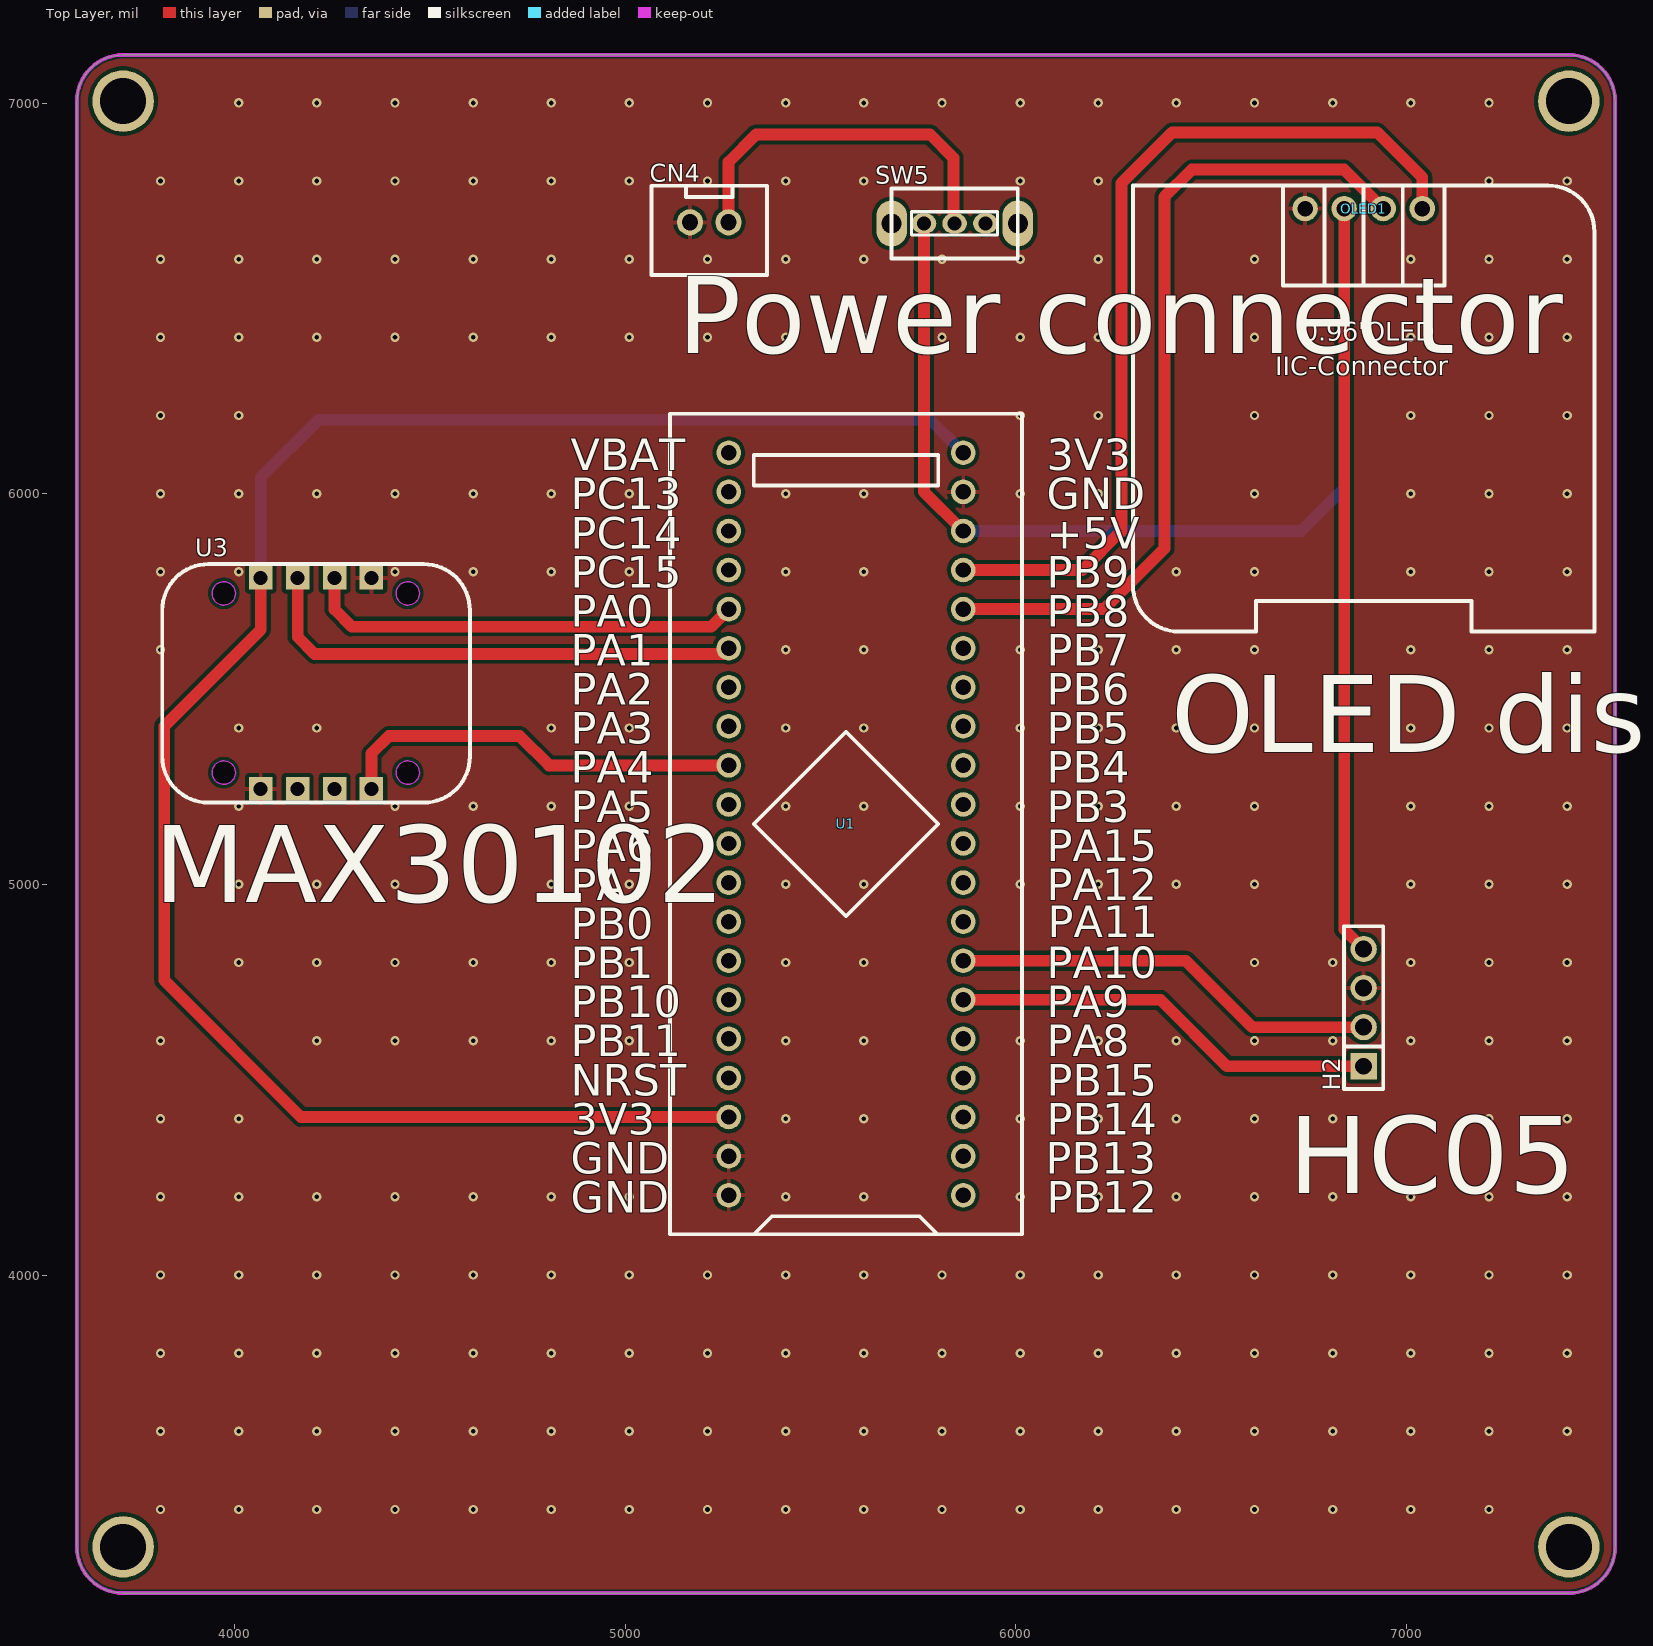
[diagram p0: Top Layer view]
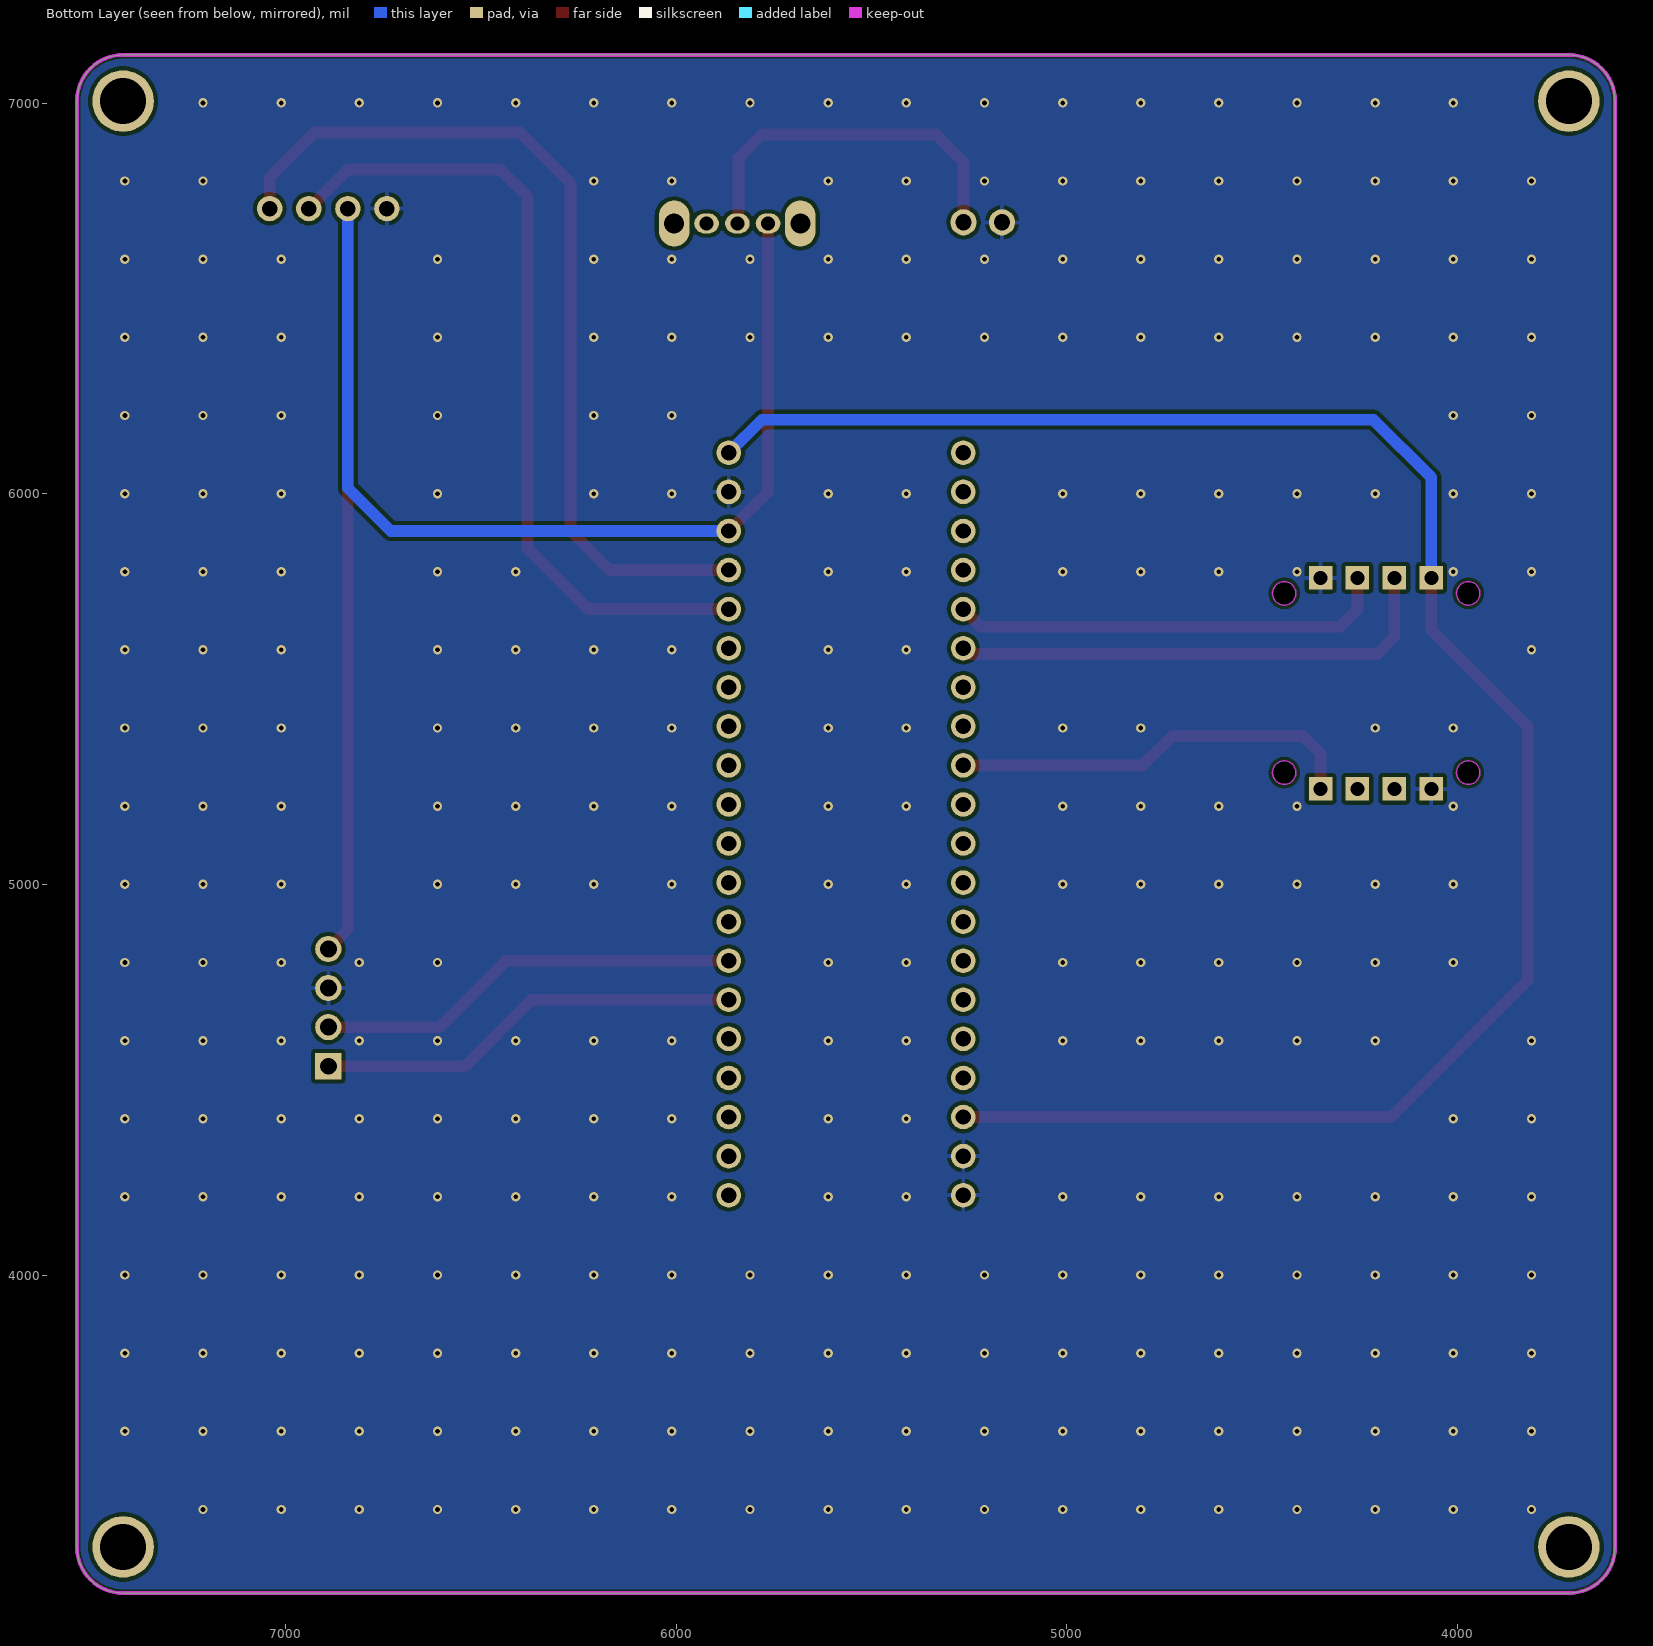
[diagram p1: Bottom Layer view, seen from below]
# Altium PCB MISC50728.pcbdoc
Units mil, origin at the board's own origin, x right, y up, seen from the top; angles counter-clockwise.
Board outline 3937.01 x 3937.01 mil, 2 copper layers (Top Layer, Bottom Layer), stack 62.206 mil thick; 6 components, 38 nets, 67 pads, 286 vias.

## Layer stack, top to bottom
Top Solder Mask Layer: solder mask 0.394, Dk 3.3
Top Layer: signal copper 1.379
Dielectric1: surface 59.449, FR4, Dk 4.5
Bottom Layer: signal copper 1.378
Bottom Solder Mask Layer: solder mask 0.394, Dk 3.3

## Board outline
3714.61,7123.5 ccw(c3714.61,7005.39) 3596.5,7005.39 3596.5,3304.61 ccw(c3714.61,3304.61) 3714.61,3186.5 7415.39,3186.5 ccw(c7415.39,3304.61) 7533.5,3304.61 7533.5,7005.39 ccw(c7415.39,7005.39) 7415.39,7123.5 3714.61,7123.5

## Design rules (kind name [scope] priority, off if disabled: settings)
BoardOutlineClearance copperThickness2oz_1 [All] p2 off: genericclearance=7.99 ignorepadtopadclearanceinfootprint=FALSE except(0: Arc-SplitContinuation Track-SplitContinuation SMDPad-SplitContinuation THPad-SplitContinuation Via-SplitContinuation Fill-SplitContinuation Region-SplitContinuation Poly-SplitContinuation Text-SplitContinuation Hole-SplitContinuation; 5.98: Arc-CutoutEdge Track-CutoutEdge SMDPad-CutoutEdge THPad-CutoutEdge Via-CutoutEdge Text-CutoutEdge; 6.9: Hole-OutlineEdge Hole-CutoutEdge; 10: Poly-OutlineEdge Poly-CutoutEdge; 11.81: Arc-OutlineEdge Track-OutlineEdge SMDPad-OutlineEdge THPad-OutlineEdge Via-OutlineEdge Fill-OutlineEdge Region-OutlineEdge Text-OutlineEdge Fill-CutoutEdge Region-CutoutEdge)
BoardOutlineClearance Plane_innerPlane_1 [All] p4 off: genericclearance=4.02 ignorepadtopadclearanceinfootprint=FALSE except(0: Arc-SplitContinuation Track-SplitContinuation SMDPad-SplitContinuation THPad-SplitContinuation Via-SplitContinuation Fill-SplitContinuation Region-SplitContinuation Poly-SplitContinuation Text-SplitContinuation Hole-SplitContinuation; 5.98: Arc-CutoutEdge Track-CutoutEdge SMDPad-CutoutEdge THPad-CutoutEdge Via-CutoutEdge Text-CutoutEdge; 6.9: Hole-OutlineEdge Hole-CutoutEdge; 10: Poly-OutlineEdge Poly-CutoutEdge; 11.81: Arc-OutlineEdge Track-OutlineEdge SMDPad-OutlineEdge THPad-OutlineEdge Via-OutlineEdge Fill-OutlineEdge Region-OutlineEdge Text-OutlineEdge Fill-CutoutEdge Region-CutoutEdge)
BoardOutlineClearance Copper_copperRegion_1 [All] p6 off: genericclearance=4.02 ignorepadtopadclearanceinfootprint=FALSE except(0: Arc-SplitContinuation Track-SplitContinuation SMDPad-SplitContinuation THPad-SplitContinuation Via-SplitContinuation Fill-SplitContinuation Region-SplitContinuation Poly-SplitContinuation Text-SplitContinuation Hole-SplitContinuation; 5.98: Arc-CutoutEdge Track-CutoutEdge SMDPad-CutoutEdge THPad-CutoutEdge Via-CutoutEdge Text-CutoutEdge; 6.9: Hole-OutlineEdge Hole-CutoutEdge; 10: Poly-OutlineEdge Poly-CutoutEdge; 11.81: Arc-OutlineEdge Track-OutlineEdge SMDPad-OutlineEdge THPad-OutlineEdge Via-OutlineEdge Fill-OutlineEdge Region-OutlineEdge Text-OutlineEdge Fill-CutoutEdge Region-CutoutEdge)
BoardOutlineClearance copperThickness1oz_1 [All] p8: genericclearance=4.02 ignorepadtopadclearanceinfootprint=FALSE except(0: Arc-SplitContinuation Track-SplitContinuation SMDPad-SplitContinuation THPad-SplitContinuation Via-SplitContinuation Fill-SplitContinuation Region-SplitContinuation Poly-SplitContinuation Text-SplitContinuation Hole-SplitContinuation; 5.98: Arc-CutoutEdge Track-CutoutEdge SMDPad-CutoutEdge THPad-CutoutEdge Via-CutoutEdge Text-CutoutEdge; 6.9: Hole-OutlineEdge Hole-CutoutEdge; 10: Poly-OutlineEdge Poly-CutoutEdge; 11.81: Arc-OutlineEdge Track-OutlineEdge SMDPad-OutlineEdge THPad-OutlineEdge Via-OutlineEdge Fill-OutlineEdge Region-OutlineEdge Text-OutlineEdge Fill-CutoutEdge Region-CutoutEdge)
Clearance copperThickness2oz [All] p1 off: gap=7.99 ignorepadtopadclearanceinfootprint=FALSE except(5.98: SMDPad-Track SMDPad-SMDPad THPad-Track SMDPad-THPad THPad-THPad Track-Via SMDPad-Via THPad-Via Via-Via Fill-SMDPad Region-SMDPad Fill-THPad Region-THPad Fill-Via Region-Via Fill-Fill Fill-Region Region-Region Arc-Track Arc-SMDPad Arc-THPad Arc-Via Fill-Arc Region-Arc Arc-Arc Text-Track SMDPad-Text Text-THPad Text-Via Fill-Text Region-Text Arc-Text Text-Text; 6.9: Hole-Track Hole-SMDPad Hole-THPad Hole-Via Fill-Hole Region-Hole Hole-Arc Hole-Text; 10: Poly-Track Poly-SMDPad Poly-THPad Poly-Via Poly-Fill Poly-Region Poly-Poly Poly-Arc Poly-Text Poly-Hole; 11.81: Fill-Track Region-Track)
Clearance Plane_innerPlane [All] p3 off: gap=4.02 ignorepadtopadclearanceinfootprint=FALSE except(5.98: SMDPad-Track SMDPad-SMDPad THPad-Track SMDPad-THPad THPad-THPad Track-Via SMDPad-Via THPad-Via Via-Via Fill-SMDPad Region-SMDPad Fill-THPad Region-THPad Fill-Via Region-Via Fill-Fill Fill-Region Region-Region Arc-Track Arc-SMDPad Arc-THPad Arc-Via Fill-Arc Region-Arc Arc-Arc Text-Track SMDPad-Text Text-THPad Text-Via Fill-Text Region-Text Arc-Text Text-Text; 6.9: Hole-Track Hole-SMDPad Hole-THPad Hole-Via Fill-Hole Region-Hole Hole-Arc Hole-Text; 10: Poly-Track Poly-SMDPad Poly-THPad Poly-Via Poly-Fill Poly-Region Poly-Poly Poly-Arc Poly-Text Poly-Hole; 11.81: Fill-Track Region-Track)
Clearance Copper_copperRegion [All] p5 off: gap=4.02 ignorepadtopadclearanceinfootprint=FALSE except(5.98: SMDPad-Track SMDPad-SMDPad THPad-Track SMDPad-THPad THPad-THPad Track-Via SMDPad-Via THPad-Via Via-Via Fill-SMDPad Region-SMDPad Fill-THPad Region-THPad Fill-Via Region-Via Fill-Fill Fill-Region Region-Region Arc-Track Arc-SMDPad Arc-THPad Arc-Via Fill-Arc Region-Arc Arc-Arc Text-Track SMDPad-Text Text-THPad Text-Via Fill-Text Region-Text Arc-Text Text-Text; 6.9: Hole-Track Hole-SMDPad Hole-THPad Hole-Via Fill-Hole Region-Hole Hole-Arc Hole-Text; 10: Poly-Track Poly-SMDPad Poly-THPad Poly-Via Poly-Fill Poly-Region Poly-Poly Poly-Arc Poly-Text Poly-Hole; 11.81: Fill-Track Region-Track)
Clearance copperThickness1oz [All] p7: gap=4.02 ignorepadtopadclearanceinfootprint=FALSE except(5.98: SMDPad-Track SMDPad-SMDPad THPad-Track SMDPad-THPad THPad-THPad Track-Via SMDPad-Via THPad-Via Via-Via Fill-SMDPad Region-SMDPad Fill-THPad Region-THPad Fill-Via Region-Via Fill-Fill Fill-Region Region-Region Arc-Track Arc-SMDPad Arc-THPad Arc-Via Fill-Arc Region-Arc Arc-Arc Text-Track SMDPad-Text Text-THPad Text-Via Fill-Text Region-Text Arc-Text Text-Text; 6.9: Hole-Track Hole-SMDPad Hole-THPad Hole-Via Fill-Hole Region-Hole Hole-Arc Hole-Text; 10: Poly-Track Poly-SMDPad Poly-THPad Poly-Via Poly-Fill Poly-Region Poly-Poly Poly-Arc Poly-Text Poly-Hole; 11.81: Fill-Track Region-Track)
DiffPairsRouting differentialPair [All] p1: maxlimit=6 minlimit=6 mostfreqgap=6 toplayer_minwidth=5 toplayer_prefwidth=10 toplayer_maxwidth=100 toplayer_mingap=6 toplayer_prefgap=6 toplayer_maxgap=6 bottomlayer_minwidth=5 bottomlayer_prefwidth=10 bottomlayer_maxwidth=100 bottomlayer_mingap=6 bottomlayer_prefgap=6 bottomlayer_maxgap=6 maxuncoupledlength=10
HoleToHoleClearance otherClearance [All] p1: gap=11.81 allowstackedmicrovias=TRUE
Length netLength [All] p1: minlimit=0 maxlimit=0
PasteMaskExpansion pasteMaskExpansion [All] p1: expansion=0
PlaneConnect innerPlane [All] p1: planeconnectstyle=Relief reliefexpansion=20 reliefentries=4 reliefconductorwidth=10 reliefairgap=10
PolygonConnect copperRegion [All] p1: connectstyle=Relief reliefconductorwidth=10 reliefentries=4 polygonreliefangle="90 Angle" airgapwidth=10 via.connectstyle=Relief via.reliefconductorwidth=10 via.reliefentries=4 via.polygonreliefangle="90 Angle" via.airgapwidth=10
RoutingVias viaSize [All] p1: holewidth=12.01 width=24.02 viastyle="Through Hole" minholewidth=11.81 minwidth=19.68 maxholewidth=248.03 maxwidth=393.7
SolderMaskExpansion solderMaskExpansion [IsVia] p1: expansion=-1000 istentingtop=TRUE
SolderMaskExpansion solderMaskExpansion [All] p2: expansion=2 istentingtop=FALSE
Width copperThickness2oz_2 [All] p1 off: maxlimit=100 minlimit=8 preferedwidth=10
Width copperThickness1oz_2 [All] p2: maxlimit=100 minlimit=5 preferedwidth=10

## Components (designator, comment, footprint, x,y, rotation, side; value= is the part's Value field where it differs from the comment)
CN4 "XH2.54*2P_THT" CONN-TH_2P-P2.50-XH2.54-2P 5215,6695 r0 top
H2 "" HDR-TH_4P-P2.54-V-F 6890,4685 r90 top
OLED1 "" 0.96OLED_4P 6890,6730 r0 top
SW5 "" 拨动开关 5837.9,6692.05 r0 top
U1 "STM32F103C8T6-Card" CONN-TH_L53.3-W22.9_STM32F103C8T6-CARD 5565,5155 r90 top
U3 "MAX30102" MAX30102 3815,5820 r0 top

## Footprints (in the part's own frame and the unit in brackets; to place one, negate y for a bottom-side part, rotate by r counter-clockwise, add the part's x,y. Pads: shape width x height; smd on the part's side, far side on the other; paste and mask are expansions set on the pad)
0.96OLED_4P [mm]
  round 1.65 hole 1 copper offset 0,0: 1(-3.81,-0.001) 2(-1.27,0.002) 3(1.27,0.002) 4(3.81,0.002)
  silkscreen extent -15,-27.5 15,1.5
CONN-TH_2P-P2.50-XH2.54-2P [mm]
  round 1.7 hole 1.05 paste+0 mask+0.05: 1(1.25,0) 2(-1.25,0)
  silkscreen extent -3.75,-3.42 3.75,2.37
CONN-TH_L53.3-W22.9_STM32F103C8T6-CARD [mm]
  round 1.6 hole 1: 1(-24.13,-7.62) 2(-21.59,-7.62) 3(-19.05,-7.62) 4(-16.51,-7.62) 5(-13.97,-7.62) 6(-11.43,-7.62) 7(-8.89,-7.62) 8(-6.35,-7.62) 9(-3.81,-7.62) 10(-1.27,-7.62) 11(1.27,-7.62) 12(3.81,-7.62) 13(6.35,-7.62) 14(8.89,-7.62) 15(11.43,-7.62) 16(13.97,-7.62) 17(16.51,-7.62) 18(19.05,-7.62) 19(21.59,-7.62) 20(24.13,-7.62) 21(24.13,7.62) 22(21.59,7.62) 23(19.05,7.62) 24(16.51,7.62) 25(13.97,7.62) 26(11.43,7.62) 27(8.89,7.62) 28(6.35,7.62) 29(3.81,7.62) 30(1.27,7.62) 31(-1.27,7.62) 32(-3.81,7.62) 33(-6.35,7.62) 34(-8.89,7.62) 35(-11.43,7.62) 36(-13.97,7.62) 37(-16.51,7.62) 38(-19.05,7.62) 39(-21.59,7.62) 40(-24.13,7.62)
  silkscreen extent -26.67,-11.43 26.67,11.43
HDR-TH_4P-P2.54-V-F [mm]
  rect 1.7x1.7 hole 1.1: 1(-3.81,0)
  round 1.7 hole 1.1: 2(-1.27,0) 3(1.27,0) 4(3.81,0)
  silkscreen extent -5.29,-1.27 5.29,1.27
MAX30102 [mil]
  rect 60x60 hole 36: 1(251.97,-35) 2(346.46,-35) 3(440.94,-35) 4(535.43,-35) 5(251.97,-575) 6(346.46,-575) 7(440.94,-575) 8(535.43,-575)
  Board Outline Layer circle w0.1: c157.48,-74.8 r30
  Board Outline Layer circle w0.1: c157.48,-533.46 r30
  Board Outline Layer circle w0.1: c628.5,-74.8 r30
  Board Outline Layer circle w0.1: c628.5,-533.46 r30
  Board Outline Layer region: 187.48,-74.8 184.51,-87.82 176.18,-98.26 164.16,-104.05 150.8,-104.05 138.78,-98.26 130.45,-87.82 127.48,-74.8 127.48,-74.8 130.45,-61.79 138.78,-51.35 150.8,-45.56 164.16,-45.56 176.18,-51.35 184.51,-61.79 187.48,-74.8
  Board Outline Layer region: 187.48,-74.8 187.11,-79.5 186.01,-84.07 184.21,-88.42 181.75,-92.44 178.69,-96.02 175.11,-99.07 171.1,-101.53 166.75,-103.33 162.17,-104.43 157.48,-104.8 152.79,-104.43 148.21,-103.33 143.86,-101.53 139.85,-99.07 136.27,-96.02 133.21,-92.44 130.75,-88.42 128.95,-84.07 127.85,-79.5 127.48,-74.8 127.85,-70.11 128.95,-65.53 130.75,-61.18 133.21,-57.17 136.27,-53.59 139.85,-50.53 143.86,-48.07 148.21,-46.27 152.79,-45.17 157.48,-44.8 162.17,-45.17 166.75,-46.27 171.1,-48.07 175.11,-50.53 178.69,-53.59 181.75,-57.17 184.21,-61.18 186.01,-65.53 187.11,-70.11
  Board Outline Layer region: 187.48,-533.46 184.51,-546.48 176.18,-556.92 164.16,-562.71 150.8,-562.71 138.78,-556.92 130.45,-546.48 127.48,-533.46 127.48,-533.46 130.45,-520.45 138.78,-510.01 150.8,-504.22 164.16,-504.22 176.18,-510.01 184.51,-520.45 187.48,-533.46
  Board Outline Layer region: 187.48,-533.46 187.11,-538.16 186.01,-542.74 184.21,-547.08 181.75,-551.1 178.69,-554.68 175.11,-557.74 171.1,-560.19 166.75,-562 162.17,-563.1 157.48,-563.46 152.79,-563.1 148.21,-562 143.86,-560.19 139.85,-557.74 136.27,-554.68 133.21,-551.1 130.75,-547.08 128.95,-542.74 127.85,-538.16 127.48,-533.46 127.85,-528.77 128.95,-524.19 130.75,-519.84 133.21,-515.83 136.27,-512.25 139.85,-509.19 143.86,-506.73 148.21,-504.93 152.79,-503.83 157.48,-503.46 162.17,-503.83 166.75,-504.93 171.1,-506.73 175.11,-509.19 178.69,-512.25 181.75,-515.83 184.21,-519.84 186.01,-524.19 187.11,-528.77
  Board Outline Layer region: 658.5,-74.8 655.53,-87.82 647.21,-98.26 635.18,-104.05 621.83,-104.05 609.8,-98.26 601.47,-87.82 598.5,-74.8 598.5,-74.8 601.47,-61.79 609.8,-51.35 621.83,-45.56 635.18,-45.56 647.21,-51.35 655.53,-61.79 658.5,-74.8
  Board Outline Layer region: 658.5,-74.8 658.13,-79.5 657.04,-84.07 655.23,-88.42 652.77,-92.44 649.72,-96.02 646.14,-99.07 642.12,-101.53 637.77,-103.33 633.2,-104.43 628.5,-104.8 623.81,-104.43 619.23,-103.33 614.88,-101.53 610.87,-99.07 607.29,-96.02 604.23,-92.44 601.77,-88.42 599.97,-84.07 598.87,-79.5 598.5,-74.8 598.87,-70.11 599.97,-65.53 601.77,-61.18 604.23,-57.17 607.29,-53.59 610.87,-50.53 614.88,-48.07 619.23,-46.27 623.81,-45.17 628.5,-44.8 633.2,-45.17 637.77,-46.27 642.12,-48.07 646.14,-50.53 649.72,-53.59 652.77,-57.17 655.23,-61.18 657.04,-65.53 658.13,-70.11
  Board Outline Layer region: 658.5,-533.46 655.53,-546.48 647.21,-556.92 635.18,-562.71 621.83,-562.71 609.8,-556.92 601.47,-546.48 598.5,-533.46 598.5,-533.46 601.47,-520.45 609.8,-510.01 621.83,-504.22 635.18,-504.22 647.21,-510.01 655.53,-520.45 658.5,-533.46
  Board Outline Layer region: 658.5,-533.46 658.13,-538.16 657.04,-542.74 655.23,-547.08 652.77,-551.1 649.72,-554.68 646.14,-557.74 642.12,-560.19 637.77,-562 633.2,-563.1 628.5,-563.46 623.81,-563.1 619.23,-562 614.88,-560.19 610.87,-557.74 607.29,-554.68 604.23,-551.1 601.77,-547.08 599.97,-542.74 598.87,-538.16 598.5,-533.46 598.87,-528.77 599.97,-524.19 601.77,-519.84 604.23,-515.83 607.29,-512.25 610.87,-509.19 614.88,-506.73 619.23,-504.93 623.81,-503.83 628.5,-503.46 633.2,-503.83 637.77,-504.93 642.12,-506.73 646.14,-509.19 649.72,-512.25 652.77,-515.83 655.23,-519.84 657.04,-524.19 658.13,-528.77
  Multi-Layer board cut-out: 187.48,-74.8 184.51,-87.82 176.18,-98.26 164.16,-104.05 150.8,-104.05 138.78,-98.26 130.45,-87.82 127.48,-74.8 127.48,-74.8 130.45,-61.79 138.78,-51.35 150.8,-45.56 164.16,-45.56 176.18,-51.35 184.51,-61.79 187.48,-74.8
  Multi-Layer board cut-out: 187.48,-533.46 184.51,-546.48 176.18,-556.92 164.16,-562.71 150.8,-562.71 138.78,-556.92 130.45,-546.48 127.48,-533.46 127.48,-533.46 130.45,-520.45 138.78,-510.01 150.8,-504.22 164.16,-504.22 176.18,-510.01 184.51,-520.45 187.48,-533.46
  Multi-Layer board cut-out: 658.5,-74.8 655.53,-87.82 647.21,-98.26 635.18,-104.05 621.83,-104.05 609.8,-98.26 601.47,-87.82 598.5,-74.8 598.5,-74.8 601.47,-61.79 609.8,-51.35 621.83,-45.56 635.18,-45.56 647.21,-51.35 655.53,-61.79 658.5,-74.8
  Multi-Layer board cut-out: 658.5,-533.46 655.53,-546.48 647.21,-556.92 635.18,-562.71 621.83,-562.71 609.8,-556.92 601.47,-546.48 598.5,-533.46 598.5,-533.46 601.47,-520.45 609.8,-510.01 621.83,-504.22 635.18,-504.22 647.21,-510.01 655.53,-520.45 658.5,-533.46
  silkscreen extent 0,-610 787,0
拨动开关 [mil]
  oval 63x51.2 hole 35.4 paste+0 mask+2: 1(-73.4,0) 2(5,0) 3(84,0)
  oval 78.7x118.1 hole 51.2 paste+0 mask+2: 4(166.7,0) 5(-156.1,0)
  silkscreen extent -156,-90 167,90

## Free pads (board coordinates)
  round 157.48 hole 118.11: 1(3714.61,7005.39) 1(3714.61,3304.61) 1(7415.39,7005.39) 1(7415.39,3304.61)

## Via types
v1: diameter 24.02, hole 12, Top Layer to Bottom Layer, 286 vias

## Nets (pads, with @x,y where several pads share a name; then routed paths per layer and width w, separated by ;. In a path a pad name is that pad's centre, name@x,y a point inside that pad or via, vN(x,y) a via of type N, cw(c..) or ccw(c..) an arc to the next point about the centre after c; other vN are vias at no path point)
$1N17118: CN4.1 SW5.2 | length 953.3
  Top Layer w30: CN4.1 5264.22,6849.22 5335,6920 5780,6920 5840,6860 5840,6694.95 SW5.2
+5V: H2.4 OLED1.2 SW5.1 U1.18 | length 4480
  Top Layer w30: SW5.1 5764.5,6005.5 U1.18 ; OLED1.2@6840,6730.05 6840,4885 H2.4
  Bottom Layer w30: U1.18 6730,5905 6840,6015 OLED1.2@6840,6730.05
GND: CN4.2 H2.3 OLED1.1 U1.19 U1.39 U1.40 U3.4 U3.5
  other v1: 3810.6,3400.6 4010.6,3400.6 4210.6,3400.6 4410.6,3400.6 4610.6,3400.6 4810.6,3400.6 5010.6,3400.6 5210.6,3400.6 5410.6,3400.6 5610.6,3400.6 5810.6,3400.6 6010.6,3400.6 6210.6,3400.6 6410.6,3400.6 6610.6,3400.6 6810.6,3400.6 7010.6,3400.6 7210.6,3400.6 3810.6,3600.6 4010.6,3600.6 4210.6,3600.6 4410.6,3600.6 4610.6,3600.6 4810.6,3600.6 5010.6,3600.6 5210.6,3600.6 5410.6,3600.6 5610.6,3600.6 5810.6,3600.6 6010.6,3600.6 6210.6,3600.6 6410.6,3600.6 6610.6,3600.6 6810.6,3600.6 7010.6,3600.6 7210.6,3600.6 7410.6,3600.6 3810.6,3800.6 4010.6,3800.6 4210.6,3800.6 4410.6,3800.6 4610.6,3800.6 4810.6,3800.6 5010.6,3800.6 5210.6,3800.6 5410.6,3800.6 5610.6,3800.6 5810.6,3800.6 6010.6,3800.6 6210.6,3800.6 6410.6,3800.6 6610.6,3800.6 6810.6,3800.6 7010.6,3800.6 7210.6,3800.6 7410.6,3800.6 3810.6,4000.6 4010.6,4000.6 4210.6,4000.6 4410.6,4000.6 4610.6,4000.6 4810.6,4000.6 5010.6,4000.6 5210.6,4000.6 5410.6,4000.6 5610.6,4000.6 5810.6,4000.6 6010.6,4000.6 6210.6,4000.6 6410.6,4000.6 6610.6,4000.6 6810.6,4000.6 7010.6,4000.6 7210.6,4000.6 7410.6,4000.6 3810.6,4200.6 4010.6,4200.6 4210.6,4200.6 4410.6,4200.6 4610.6,4200.6 4810.6,4200.6 5010.6,4200.6 5410.6,4200.6 5610.6,4200.6 6010.6,4200.6 6210.6,4200.6 6410.6,4200.6 6610.6,4200.6 6810.6,4200.6 7010.6,4200.6 7210.6,4200.6 7410.6,4200.6 3810.6,4400.6 4010.6,4400.6 5410.6,4400.6 5610.6,4400.6 6010.6,4400.6 6210.6,4400.6 6410.6,4400.6 6610.6,4400.6 6810.6,4400.6 7010.6,4400.6 7210.6,4400.6 7410.6,4400.6 3810.6,4600.6 4210.6,4600.6 4410.6,4600.6 4610.6,4600.6 4810.6,4600.6 5010.6,4600.6 5410.6,4600.6 5610.6,4600.6 6010.6,4600.6 6210.6,4600.6 6410.6,4600.6 6610.6,4600.6 6810.6,4600.6 7010.6,4600.6 7210.6,4600.6 7410.6,4600.6 4010.6,4800.6 4210.6,4800.6 4410.6,4800.6 4610.6,4800.6 4810.6,4800.6 5010.6,4800.6 5410.6,4800.6 5610.6,4800.6 6610.6,4800.6 6810.6,4800.6 7010.6,4800.6 7210.6,4800.6 7410.6,4800.6 4010.6,5000.6 4210.6,5000.6 4410.6,5000.6 4610.6,5000.6 4810.6,5000.6 5010.6,5000.6 5410.6,5000.6 5610.6,5000.6 6010.6,5000.6 6210.6,5000.6 6410.6,5000.6 6610.6,5000.6 7010.6,5000.6 7210.6,5000.6 7410.6,5000.6 4010.6,5200.6 4410.6,5200.6 4610.6,5200.6 4810.6,5200.6 5010.6,5200.6 5410.6,5200.6 5610.6,5200.6 6010.6,5200.6 6210.6,5200.6 6410.6,5200.6 6610.6,5200.6 7010.6,5200.6 7210.6,5200.6 7410.6,5200.6 4010.6,5400.6 4210.6,5400.6 4810.6,5400.6 5010.6,5400.6 5410.6,5400.6 5610.6,5400.6 6010.6,5400.6 6210.6,5400.6 6410.6,5400.6 6610.6,5400.6 7010.6,5400.6 7210.6,5400.6 7410.6,5400.6 3810.6,5600.6 5410.6,5600.6 5610.6,5600.6 6010.6,5600.6 6210.6,5600.6 6410.6,5600.6 6610.6,5600.6 7010.6,5600.6 7210.6,5600.6 7410.6,5600.6 3810.6,5800.6 4010.6,5800.6 4410.6,5800.6 4610.6,5800.6 4810.6,5800.6 5010.6,5800.6 5410.6,5800.6 5610.6,5800.6 6410.6,5800.6 6610.6,5800.6 7010.6,5800.6 7210.6,5800.6 7410.6,5800.6 3810.6,6000.6 4010.6,6000.6 4210.6,6000.6 4410.6,6000.6 4610.6,6000.6 4810.6,6000.6 5010.6,6000.6 5410.6,6000.6 5610.6,6000.6 6010.6,6000.6 6210.6,6000.6 6610.6,6000.6 7010.6,6000.6 7210.6,6000.6 7410.6,6000.6 3810.6,6200.6 4010.6,6200.6 6010.6,6200.6 6210.6,6200.6 6610.6,6200.6 7010.6,6200.6 7210.6,6200.6 7410.6,6200.6 3810.6,6400.6 4010.6,6400.6 4210.6,6400.6 4410.6,6400.6 4610.6,6400.6 4810.6,6400.6 5010.6,6400.6 5210.6,6400.6 5410.6,6400.6 5610.6,6400.6 5810.6,6400.6 6010.6,6400.6 6210.6,6400.6 6610.6,6400.6 7010.6,6400.6 7210.6,6400.6 7410.6,6400.6 3810.6,6600.6 4010.6,6600.6 4210.6,6600.6 4410.6,6600.6 4610.6,6600.6 4810.6,6600.6 5010.6,6600.6 5210.6,6600.6 5410.6,6600.6 5610.6,6600.6 5810.6,6600.6 6010.6,6600.6 6210.6,6600.6 6610.6,6600.6 7010.6,6600.6 7210.6,6600.6 7410.6,6600.6 3810.6,6800.6 4010.6,6800.6 4210.6,6800.6 4410.6,6800.6 4610.6,6800.6 4810.6,6800.6 5010.6,6800.6 5210.6,6800.6 5410.6,6800.6 5610.6,6800.6 6010.6,6800.6 6210.6,6800.6 7210.6,6800.6 7410.6,6800.6 4010.6,7000.6 4210.6,7000.6 4410.6,7000.6 4610.6,7000.6 4810.6,7000.6 5010.6,7000.6 5210.6,7000.6 5410.6,7000.6 5610.6,7000.6 5810.6,7000.6 6010.6,7000.6 6210.6,7000.6 6410.6,7000.6 6610.6,7000.6 6810.6,7000.6 7010.6,7000.6 7210.6,7000.6
NRST: U1.37
PA0: U1.25 U3.3 | length 1126.9
  Top Layer w30: U3.3 4255.94,5704.06 4300,5660 5220,5660 U1.25
PA1: U1.26 U3.2 | length 1279.2
  Top Layer w30: U3.2 4161.46,5633.54 4205,5590 5250,5590 U1.26
PA2: U1.27
PA3: U1.28
PA4: U1.29 U3.8 | length 1054.5
  Top Layer w30: U3.8 4350.43,5335.43 4395,5380 4730,5380 4805,5305 U1.29
PA5: U1.30
PA6: U1.31
PA7: U1.32
PA8: U1.5
PA9: H2.1 U1.6 | length 1095.4
  Top Layer w30: U1.6 6370,4705 6540,4535 H2.1
PA10: H2.2 U1.7 | length 1095.4
  Top Layer w30: U1.7 6435,4805 6605,4635 H2.2
PA11: U1.8
PA12: U1.9
PA15: U1.10
PB0: U1.33
PB1: U1.34
PB3: U1.11
PB4: U1.12
PB5: U1.13
PB6: U1.14
PB7: U1.15
PB8: OLED1.3 U1.16 | length 2109.6
  Top Layer w30: U1.16 6225,5705 6380,5860 6380,6760 6450,6830 6840.05,6830 OLED1.3@6940,6730.05
PB9: OLED1.4 U1.17 | length 2287.9
  Top Layer w30: U1.17 6170,5805 6270,5905 6270,6795 6400,6925 6925,6925 7040,6810 OLED1.4@7040,6730.05
PB10: U1.35
PB11: U1.36
PB12: U1.1
PB13: U1.2
PB14: U1.3
PB15: U1.4
PC13: U1.22
PC14: U1.23
PC15: U1.24
VBAT: U1.21
VCC: U1.20 U1.38 U3.1 | length 4873.8
  Top Layer w30: U3.1 4066.97,5651.97 3820,5405 3820,4755 4170,4405 U1.38
  Bottom Layer w30: U3.1 4066.97,6041.97 4215,6190 5780,6190 U1.20
pads on no net: SW5.3 SW5.4 SW5.5 U3.6 U3.7

## Polygon pours and split planes (outlines as drawn)
GND on Bottom Layer (solid, remove dead copper, pour order 2): 3525,7245 3525,3080 7700,3080 7700,7245
GND on Top Layer (solid, remove dead copper, pour order 2): 3000,7415 3000,3000 7930,3000 7930,7415

## Keep-outs
Board Outline Layer:
  the board outline again, w10

## Silkscreen, mask and mechanical layers (free items; w line width, h text height)
Top Silkscreen Layer:
  text "Power connector" at 5135,6360 h196.85
  text "VBAT" at 4860.95,6060 h80
  text "3V3" at 6079.16,6060 h80
  text "PC13" at 4860.95,5960 h80
  text "GND" at 6079.16,5960 h80
  text "PC14" at 4860.95,5860 h80
  text "+5V" at 6079.16,5860 h80
  text "PC15" at 4860.95,5760 h80
  text "PB9" at 6079.16,5760 h80
  text "PA0" at 4860.95,5660 h80
  text "PB8" at 6079.16,5660 h80
  text "PA1" at 4860.95,5560 h80
  text "PB7" at 6079.16,5560 h80
  text "PA2" at 4860.95,5460 h80
  text "PB6" at 6079.16,5460 h80
  text "PA3" at 4860.95,5360 h80
  text "PB5" at 6079.16,5360 h80
  text "OLED display" at 6398.02,5338.96 h196.85
  text "PA4" at 4860.95,5260 h80
  text "PB4" at 6079.16,5260 h80
  text "PA5" at 4860.95,5160 h80
  text "PB3" at 6079.16,5160 h80
  text "PA6" at 4860.95,5060 h80
  text "PA15" at 6079.16,5060 h80
  text "PA7" at 4860.95,4960 h80
  text "PA12" at 6079.16,4960 h80
  text "MAX30102" at 3795,4955 h196.85
  text "PA11" at 6080.95,4865 h80
  text "PB0" at 4860.95,4860 h80
  text "PB1" at 4860.95,4760 h80
  text "PA10" at 6079.16,4760 h80
  text "PB10" at 4860.95,4660 h80
  text "PA9" at 6079.16,4660 h80
  text "PB11" at 4860.95,4560 h80
  text "PA8" at 6079.16,4560 h80
  text "NRST" at 4860.95,4460 h80
  text "PB15" at 6079.16,4460 h80
  text "3V3" at 4860.95,4360 h80
  text "PB14" at 6079.16,4360 h80
  text "GND" at 4860.95,4260 h80
  text "PB13" at 6075.95,4260 h80
  text "HC05" at 6697.92,4210 h196.85
  text "GND" at 4860.95,4160 h80
  text "PB12" at 6079.16,4160 h80